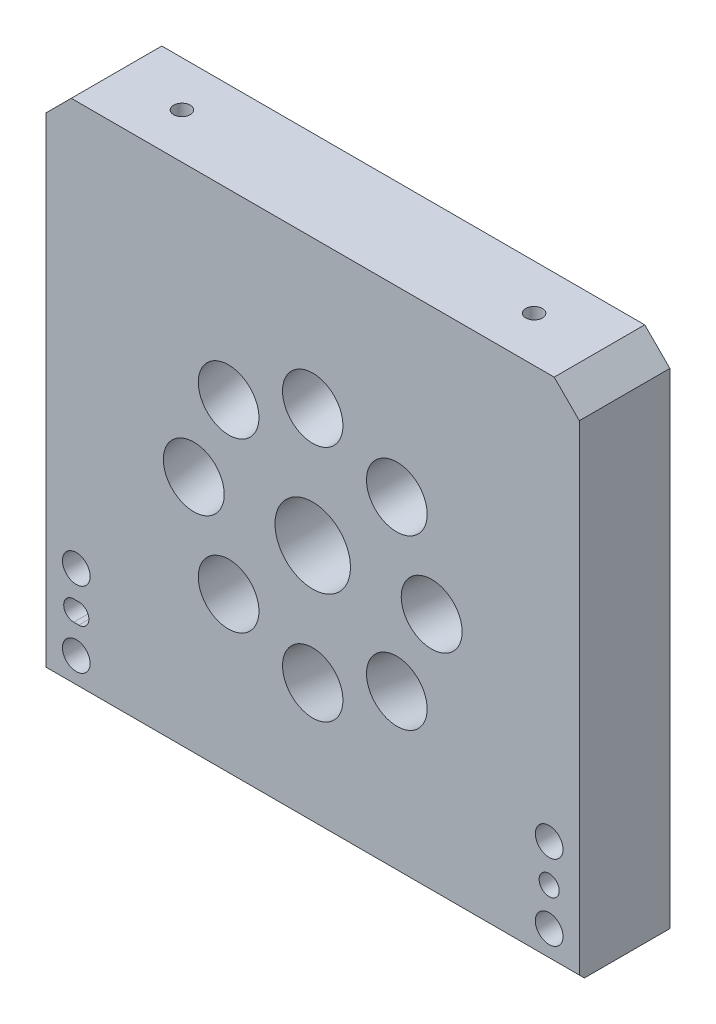
SolidWorks part; units mm, degrees
ref_plane "Front Plane" through (0, 0, 0) normal (0, 0, 1) x (1, 0, 0)
ref_plane "Top Plane" through (0, 0, 0) normal (0, 1, 0) x (1, 0, 0)
ref_plane "Right Plane" through (0, 0, 0) normal (1, 0, 0) x (0, 0, -1)
sketch "Sketch1" plane through (0, 0, 0) normal (0, 0, 1) x (1, 0, 0)
  line L1 (-53, 50.72) -> (53, 50.72)
  line L2 (-53, 50.72) -> (-53, -50.72)
  line L3 (-53, -50.72) -> (53, -50.72)
  line L4 (53, 50.72) -> (53, -50.72)
  line L5 (-53, 50.72) -> (53, -50.72) construction
  line L6 (-53, -50.72) -> (53, 50.72) construction
  point P0 (0, 0)
  dimension "D1" = 106
  dimension "D2" = 101.44
extrude "Boss-Extrude1" add sketch "Sketch1" along normal mid plane 18
sketch "Sketch3" plane through (0, 0, -9) normal (0, 0, -1) x (-1, 0, 0)
  line L1 (53, -50.72) -> (-53, -50.72) construction
  circle A0 centre (0, -2.2774) radius 7.5
  dimension "D1" = 15
  dimension "D2" = 48.4426
extrude "Cut-Extrude1" cut sketch "Sketch3" against normal through all
sketch "Sketch2" plane through (0, 0, 0) normal (1, 0, 0) x (0, 0, -1)
  line L0 (6.8631, 17.4017) -> (7.1242, 15.4188)
  line L2 (-9.7832, 21.262) -> (-9, 15.3133)
  line L3 (-9, 15.3133) -> (6.8631, 17.4017)
  line L4 (16.0472, 16.5936) -> (15.003, 24.5251)
  line L5 (15.003, 24.5251) -> (-9.7832, 21.262)
  line L6 (-9, -50.72) -> (-9, 50.72) construction
  line L9 (7.1242, 15.4188) -> (16.0472, 16.5936)
  dimension "D1" = 6
  dimension "D2" = 16
  dimension "D3" = 7.5
  dimension "D4" = 15.3133
  dimension "D5" = 8
  dimension "D6" = 25
revolve "Cut-Revolve1" cut sketch "Sketch2" angle 360 about L5
hole_wizard "M3 Tapped Hole1" positions "Sketch5" profile "Sketch4" tap size "M3" standard "Gb"
sketch "Sketch5" plane through (0, 0, -9) normal (0, 0, -1) x (-1, 0, 0)
  circle A0 centre (0, -2.2774) radius 7.5 construction
  point P0 (0, 9.1668)
  dimension "D1" = 11.4442
sketch "Sketch4" plane through (0, 9.1668, -9) normal (1, 0, 0) x (0, 1, 0)
  line L0 (0, 0) -> (0, 8.2511)
  line L1 (0, 8.2511) -> (1.25, 7.5)
  line L2 (1.25, 7.5) -> (1.25, 0)
  line L5 (1.25, 0) -> (0, 0)
  line L10 (0, 8.2511) -> (-1.25, 7.5) construction
  line L11 (0, -6.35) -> (0, 107.95) construction
  dimension "螺纹孔钻头直径" = 2.5
  dimension "螺纹孔钻头深度" = 7.5
  dimension "导头角度" = 118
cosmetic thread "Hole Thread1" parameters "D1"=6, "D2"=3
pattern_circular "CirPattern1" count 8 over 360 about axis through (0, -2.2774, 0) along (0, 0, 1) of "Cut-Revolve1", "M3 Tapped Hole1"
chamfer "Chamfer1" distance 5 angle 45 2 edges at (-53, 50.72, 0) (53, 50.72, 0)
chamfer "Chamfer2" distance 1 angle 45 1 edges at (0, -50.72, 9)
hole_wizard "Hole size per socket head cap screw type1" positions "Sketch7" profile "Sketch6" counterbore size "M5" standard "Gb" end condition through all
sketch "Sketch7" plane through (0, 0, -9) normal (0, 0, -1) x (-1, 0, 0)
  line L0 (0, 0) -> (0, -58.1524) construction
  line L2 (53, -50.72) -> (-53, -50.72) construction
  point P0 (-47, -29.72)
  point P3 (-47, -44.72)
  point P6 (47, -44.72)
  point P9 (47, -29.72)
  dimension "D1" = 94
  dimension "D2" = 15
  dimension "D3" = 6
sketch "Sketch6" plane through (47, -29.72, -9) normal (1, 0, 0) x (0, 1, 0)
  line L0 (0, 0) -> (0, 18)
  line L1 (0, 18) -> (2.75, 18)
  line L3 (2.75, 18) -> (2.75, 6)
  line L4 (2.75, 6) -> (4.75, 6)
  line L5 (4.75, 6) -> (4.75, 0)
  line L7 (4.75, 0) -> (0, 0)
  line L11 (0, -6.35) -> (0, 107.95) construction
  dimension "通孔孔直径" = 5.5
  dimension "通孔孔深度" = 18
  dimension "柱形沉头孔直径" = 9.5
  dimension "柱形沉头孔深度" = 6
hole_wizard "M4 Tapped Hole1" positions "Sketch9" profile "Sketch8" tap size "M4" standard "Gb"
sketch "Sketch9" plane through (0, 50.72, 0) normal (0, 1, 0) x (1, 0, 0)
  line L0 (0, 0) -> (0, 14.5571) construction
  point P0 (-35, 0)
  point P2 (35, 0)
  dimension "D1" = 70
sketch "Sketch8" plane through (-35, 50.72, 0) normal (1, 0, 0) x (0, 0, 1)
  line L0 (0, 0) -> (0, 13.0914)
  line L1 (0, 13.0914) -> (1.65, 12.1)
  line L2 (1.65, 12.1) -> (1.65, 0)
  line L5 (1.65, 0) -> (0, 0)
  line L10 (0, 13.0914) -> (-1.65, 12.1) construction
  line L11 (0, -6.35) -> (0, 107.95) construction
  dimension "螺纹孔钻头直径" = 3.3
  dimension "螺纹孔钻头深度" = 12.1
  dimension "导头角度" = 118
cosmetic thread "Hole Thread2" parameters "D1"=10, "D2"=4
cosmetic thread "Hole Thread3" parameters "D1"=10, "D2"=4
sketch "Sketch11" plane through (0, 0, -9) normal (0, 0, -1) x (-1, 0, 0)
  line L0 (-47, -29.72) -> (-47, -44.72) construction
  line L1 (53, -50.72) -> (-53, -50.72) construction
  line L2 (46.5, -37.22) -> (47.5, -37.22) construction
  line L3 (46.5, -35.22) -> (47.5, -35.22)
  line L4 (46.5, -39.22) -> (47.5, -39.22)
  line L5 (47, -29.72) -> (47, -44.72) construction
  circle A0 centre (-47, -37.22) radius 2
  arc A1 (46.5, -35.22) -> (46.5, -39.22) centre (46.5, -37.22) ccw
  arc A2 (47.5, -39.22) -> (47.5, -35.22) centre (47.5, -37.22) ccw
  point P10 (47, -37.22)
  dimension "D2" = 4
  dimension "D1" = 13.5
  dimension "D3" = 4
  dimension "D4" = 1
extrude "Cut-Extrude2" cut sketch "Sketch11" against normal through all
